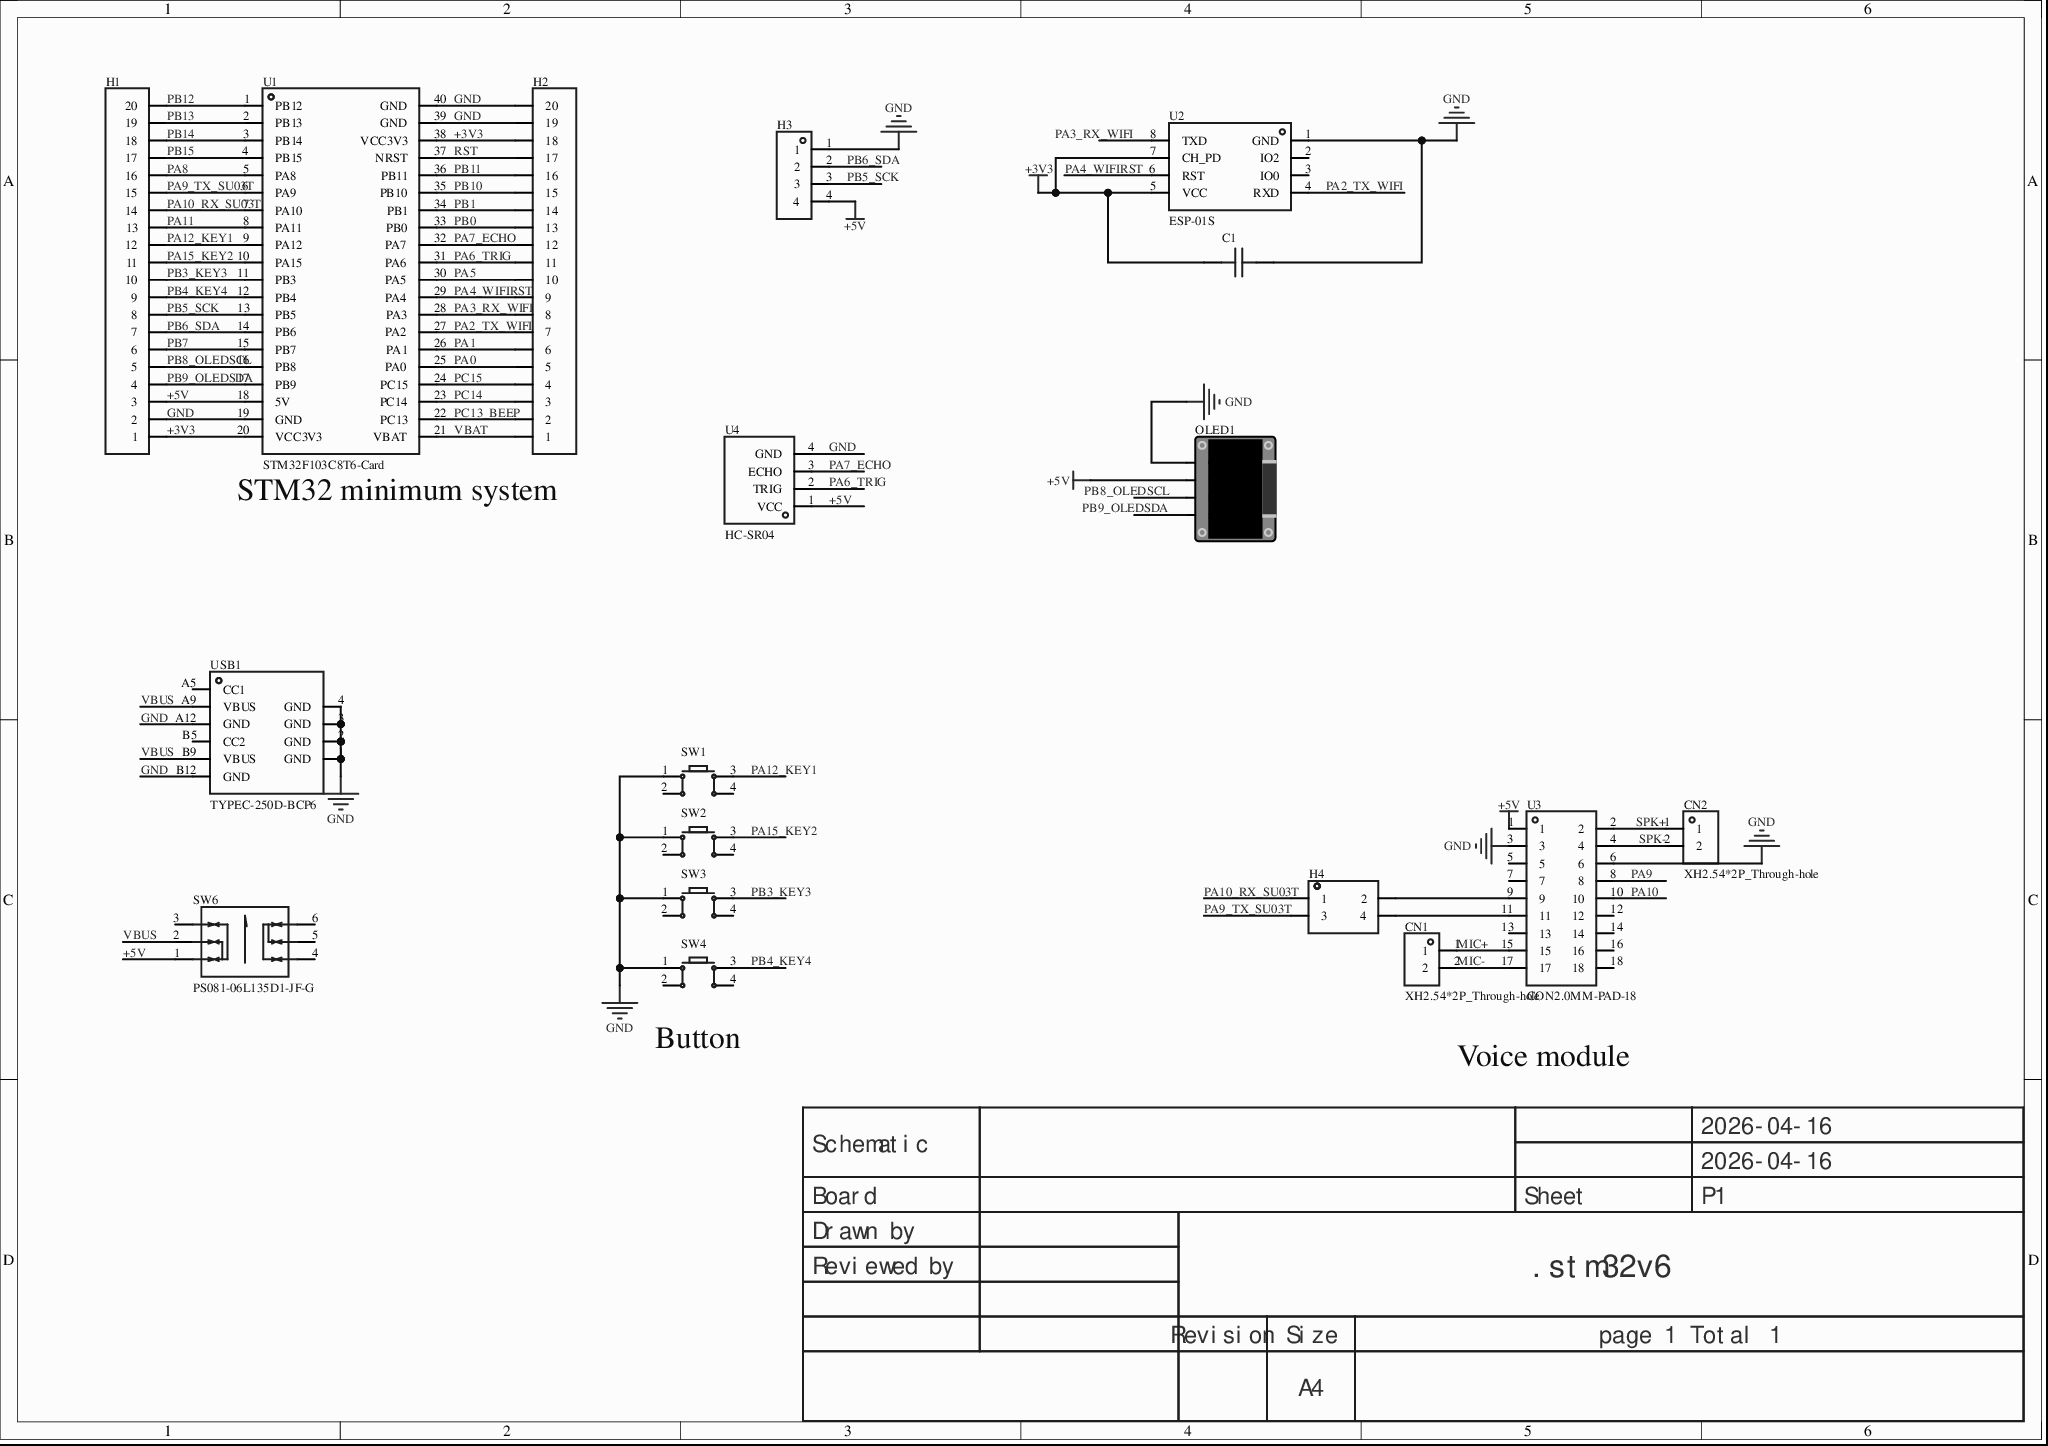
[diagram p0: MISC89113-3.schdoc]
# Altium project MISC89113-2.PrjPcb
1 sheet, 18 parts. Net scope: global (net labels, ports and power ports of the same name join across sheets).
Board file: MISC89113.pcbdoc

## Sheet MISC89113-3.schdoc
size 297 x 209 mm; Version: V1.0; @Project Name: MISC89113; @Page Count: 1; @Update Date: 2026-04-16; @Create Date: 2026-04-16; @Schematic Name: MISC89113; @Page No: 1; @Create Time: 23:22:16; @Update Time: 17:32:40; @Board Name: MISC89113

### Parts
C1  100nF  [C0603]  (value not drawn)
CN1  XH2.54*2P_Through-hole  [CONN-TH_2P-P2.50-XH2.54-2P]
CN2  XH2.54*2P_Through-hole  [CONN-TH_2P-P2.50-XH2.54-2P]
H1  (no value)  [HDR-TH_20P-P2.54-V-F]
H2  (no value)  [HDR-TH_20P-P2.54-V-F]
H3  (no value)  [HDR-TH_4P-P2.54-V-F]
H4  (no value)  [HDR-TH_4P-P2.54-V-F-R2-C2-S2.54]
OLED1  (no value)  [0.96OLED_4P]
SW1  (no value)  [SW-TH_4P-L6.0-W6.0-P4.50-LS6.5]
SW2  (no value)  [SW-TH_4P-L6.0-W6.0-P4.50-LS6.5]
SW3  (no value)  [SW-TH_4P-L6.0-W6.0-P4.50-LS6.5]
SW4  (no value)  [SW-TH_4P-L6.0-W6.0-P4.50-LS6.5]
SW6  PS081-06L135D1-JF-G  [SW-TH_6P-L8.0-W8.0-P2.50-TL]
U1  STM32F103C8T6-Card  [CONN-TH_L53.3-W22.9_STM32F103C8T6-CARD]
U2  ESP-01S  [WIFIM-TH_ESP-01S]
U3  CON2.0MM-PAD-18  [CONN-TH_18P-P2.00_C9900078766]
U4  HC-SR04  [TH_HC-SR04V]
USB1  TYPEC-250D-BCP6  [USB-C-SMD_TYPEC-250D-BCP6]

### Nets
+3V3: C1.1 H1.1 H2.18 U1.20(VCC3V3) U1.38(VCC3V3) U2.5(VCC) U2.7(CH_PD)
+5V: H1.3 H3.4 OLED1.2(VCC) SW6.1 U1.18(5V) U3.1 U4.1(VCC)
GND: C1.2 H1.2 H2.19 H2.20 H3.1 OLED1.1(GND) SW1.1 SW2.1 SW3.1 SW4.1 U1.19(GND) U1.39(GND) U1.40(GND) U2.1(GND) U3.3 U3.6 U4.4(GND) USB1.1(GND) USB1.2(GND) USB1.3(GND) USB1.4(GND) USB1.A12(GND) USB1.B12(GND)
MIC+: CN1.1 U3.15
MIC-: CN1.2 U3.17
PA0: H2.5 U1.25(PA0)
PA1: H2.6 U1.26(PA1)
PA2_TX_WIFI: H2.7 U1.27(PA2) U2.4(RXD)
PA3_RX_WIFI: H2.8 U1.28(PA3) U2.8(TXD)
PA4_WIFIRST: H2.9 U1.29(PA4) U2.6(RST)
PA5: H2.10 U1.30(PA5)
PA6_TRIG: H2.11 U1.31(PA6) U4.2(TRIG)
PA7_ECHO: H2.12 U1.32(PA7) U4.3(ECHO)
PA8: H1.16 U1.5(PA8)
PA9: U3.8
PA9_TX_SU03T: H1.15 H4.3 U1.6(PA9)
PA10: U3.10
PA10_RX_SU03T: H1.14 H4.1 U1.7(PA10)
PA11: H1.13 U1.8(PA11)
PA12_KEY1: H1.12 SW1.3 U1.9(PA12)
PA15_KEY2: H1.11 SW2.3 U1.10(PA15)
PB0: H2.13 U1.33(PB0)
PB1: H2.14 U1.34(PB1)
PB3_KEY3: H1.10 SW3.3 U1.11(PB3)
PB4_KEY4: H1.9 SW4.3 U1.12(PB4)
PB5_SCK: H1.8 H3.3 U1.13(PB5)
PB6_SDA: H1.7 H3.2 U1.14(PB6)
PB7: H1.6 U1.15(PB7)
PB8_OLEDSCL: H1.5 OLED1.3(SCL) U1.16(PB8)
PB9_OLEDSDA: H1.4 OLED1.4(SDA) U1.17(PB9)
PB10: H2.15 U1.35(PB10)
PB11: H2.16 U1.36(PB11)
PB12: H1.20 U1.1(PB12)
PB13: H1.19 U1.2(PB13)
PB14: H1.18 U1.3(PB14)
PB15: H1.17 U1.4(PB15)
PC13_BEEP: H2.2 U1.22(PC13)
PC14: H2.3 U1.23(PC14)
PC15: H2.4 U1.24(PC15)
RST: H2.17 U1.37(NRST)
SPK+: CN2.1 U3.2
SPK-: CN2.2 U3.4
VBAT: H2.1 U1.21(VBAT)
VBUS: SW6.2 USB1.A9(VBUS) USB1.B9(VBUS)
NetH4_2: H4.2 U3.9
NetH4_4: H4.4 U3.11

Not connected (* = marked no-connect by the designer): SW1 2 4; SW2 2 4; SW3 2 4; SW4 2 4; SW6 3 4 5 6; U2 2(IO2)* 3(IO0)*; U3 5 7 12 13 14 16 18; USB1 A5(CC1)* B5(CC2)*

### Notes on the sheet
- STM32 minimum system
- (near SW4) Button
- Voice module
- Labels drawn without touching a wire or pin: GND, VCC
- 2026-04-16
- Schematic
- Board
- Sheet
- P1
- Drawn by
- Reviewed by
- .stm32v6
- Revision
- Size
- A4
- page 1 Total 1

### Library data of the parts
C1 = CAP_0603: Symbol: Capacitance; ConvertToPcb: yes; ModelId: ac125912035d415993ca9572d50418b10819f05c4eef4c71ace90d822a990e87; ModelName: C0603_L1.6-W0.8-H0.8; ModelTransform: 62.992,31.496,0,0,0,0,0,0,0; Device: CAP_0603; AddInBom: yes; Supplier Footprint: 0603; FootprintName: C0603; Value: 100nF
CN1 CN2 = XH2.54*2P_直插: AddInBom: yes; ModelId: 325c595e30db4df8abe76612dd40b0fa0819f05c4eef4c71ace90d822a990e87; ModelTransform: 295.275,228.346,0,180,0,0,-0.002,-20.079,-137.795; Symbol: XH2.54*2P_Through-hole; Device: XH2.54*2P_Through-hole; LCSC Part Name: XH2.54*2P_直插; SupplierPart: C9900008615; ManufacturerPart: XH2.54*2P_直插; Supplier Footprint: XH2.54_2P; JLCPCB Part Class: Extended Part; Supplier: LCSC; ConvertToPcb: yes; FootprintName: CONN-TH_2P-P2.50-XH2.54-2P; ModelName: CONN-TH_2P-P2.50-XH2.54-2P
H1 H2 = HDR-F_2.54_1x20P: ConvertToPcb: yes; ModelId: db7015f7ad9d48b8a3b1188db02e3429; ModelName: HDR-F-2.54_1x20; ModelTransform: 1999.996,100,0,0,0,0,0,0,-118.11; Symbol: HDR-F_2.54_1x20P; Device: HDR-F_2.54_1x20P; AddInBom: yes; SupplierPart: C50984; Supplier Footprint: 插件; FootprintName: HDR-TH_20P-P2.54-V-F
H3 = HDR-F_2.54_1x4P: Symbol: 2.54-1*4P female; ConvertToPcb: yes; ModelId: d187812051054f85879fcaa51a310d8e0819f05c4eef4c71ace90d822a990e87; ModelTransform: 419.6842,98.464,0,0,0,0,0,0,-118.11; Device: HDR-F_2.54_1x4P; AddInBom: yes; SupplierPart: C2718488; Supplier Footprint: 插件; FootprintName: HDR-TH_4P-P2.54-V-F; ModelName: HDR-TH_4P-P2.54-V-F
H4 = HDR-F_2.54_2x2: Symbol: HDR-F-2.54_2x2; ConvertToPcb: yes; ModelId: 870c884146ee4765973edc845f10b7af0819f05c4eef4c71ace90d822a990e87; ModelName: HDR-TH_4P-P2.54-F-LI-2X2P; ModelTransform: 215.7476,196.85,0,0,0,0,0,0,-118.11; Device: HDR-F_2.54_2x2; AddInBom: yes; SupplierPart: C92273; Supplier Footprint: 插件; FootprintName: HDR-TH_4P-P2.54-V-F-R2-C2-S2.54
OLED1 = 0.96OLED模块_4P: Symbol: 0.96OLED module_4P; ConvertToPcb: yes; ModelId: 79c000fdb68d45a296c2e9bedf4f9055; ModelTransform: 1393.69792,1318.895,0,0,0,0,0,-560.079,-137.795; Device: 0.96OLED module_4P; AddInBom: yes; FootprintName: 0.96OLED_4P; Supplier Footprint: 插件; ModelName: 0.96OLED_4P
SW1-SW4 = Key_TH_6x6x6: Contact current: 50mA; rated voltage (DC): 12V; insulation resistance: 100MΩ; circuit structure: SPST; mounting: through-hole; button shape: round button; button/cap color: black; actuating force: 260gf@±30gf; operating temperature: -25℃~+70℃; pin style: PC pin; switch length: 6mm; switch width: 6mm; switch height: 6mm; with bracket: no;; Symbol: Tactile push button; AddInBom: yes; ModelId: 20eee248bc684ccd8cbdbb1d0d91ec6f0819f05c4eef4c71ace90d822a990e87; ModelName: SW-TH_4P-L6.0-W6.0-H5.0-LS6.5-P4.50; ModelTransform: 236.22,323.03,0,90,0,0,0,0,-137.795; Device: Key_TH_6x6x6; ConvertToPcb: yes; FootprintName: SW-TH_4P-L6.0-W6.0-P4.50-LS6.5; Supplier Footprint: 插件
SW6 = PS081-06L135D1-JF-G: Circuit structure: DPDT; self-lock/no-lock: self-lock; mounting: through-hole; contact current: 100mA; rated voltage: 30V;; Manufacturer: Khon(康宏电子); AddInBom: yes; ModelId: 81096a2982954f00b80aabbc3df69c720819f05c4eef4c71ace90d822a990e87; ModelTransform: 314.96394,314.96,0,90,0,0,0,0,-137.795; Actuator/Cap Color: Blue; Symbol: PS081-06L135D1-JF-G; Device: PS081-06L135D1-JF-G; LCSC Part Name: 8x8自锁开关; SupplierPart: C46533676; ManufacturerPart: PS081-06L135D1-JF-G; Supplier Footprint: DIP-6P,8x8mm; JLCPCB Part Class: Extended Part; Datasheet: https://item.szlcsc.com/datasheet/PS081-06L135D1-JF-G/48661190.html; Supplier: LCSC; ConvertToPcb: yes; FootprintName: SW-TH_6P-L8.0-W8.0-P2.50-TL; ModelName: SW-TH_6P-L8.0-W8.0-P2.50-TL; Circuit: DPDT; Self Lock / No Lock: Self-lock; Mounting Type: Through-hole; Contact Current: 100mA; Voltage Rating: 30V; Termination Style: PC pin; Operating Temperature: -25℃~+70℃
U1 = STM32F103C8T6-Card: AddInBom: yes; Symbol: STM32F103C8T6-CARD; Device: STM32F103C8T6-Card; LCSC Part Name: STM32F103C8T6-Card; SupplierPart: C9900077949; ManufacturerPart: STM32F103C8T6-Card; Supplier Footprint: 插件; Supplier: LCSC; ConvertToPcb: yes; FootprintName: CONN-TH_L53.3-W22.9_STM32F103C8T6-CARD
U2 = ESP-01S_C111009: AddInBom: yes; ModelId: eb7175da78ae48b3b1568cfe3027405f0819f05c4eef4c71ace90d822a990e87; ModelTransform: 582.676,976.37608,0,0,0,0,0,388.346,-118.11; Symbol: ESP-01S; Device: ESP-01S_C111009; LCSC Part Name: ESP-01S; SupplierPart: C111009; ManufacturerPart: ESP-01S; Supplier Footprint: -; JLCPCB Part Class: Extended Part; Supplier: LCSC; ConvertToPcb: yes; FootprintName: WIFIM-TH_ESP-01S; ModelName: WIFIM-TH_ESP-01S
U3 = CON2.0MM-PAD-18: AddInBom: yes; ModelId: 07100c6dd3a4442ea12d6f5a4e41c4c80819f05c4eef4c71ace90d822a990e87; ModelTransform: 787.7937,374.015,0,0,0,0,0,-14.961,-118.11; Symbol: CON2.0MM-PAD-18; Device: CON2.0MM-PAD-18; LCSC Part Name: CON2.0MM-PAD-18; SupplierPart: C9900078766; ManufacturerPart: CON2.0MM-PAD-18; Supplier Footprint: TH-2*9P-2.0; JLCPCB Part Class: Extended Part; Supplier: LCSC; ConvertToPcb: yes; FootprintName: CONN-TH_18P-P2.00_C9900078766; ModelName: CONN-TH_18P-P2.00_C9900078766
U4 = HC-SR04: Manufacturer: Universal Microelectronics; AddInBom: yes; Symbol: HC-SR04; Device: HC-SR04; LCSC Part Name: HC-SR04; SupplierPart: C19857336; ManufacturerPart: HC-SR04; Supplier Footprint: -; JLCPCB Part Class: Extended part; Datasheet: https://atta.szlcsc.com/upload/public/pdf/source/20240122/47B8E374E428935B7962A2189EF91AAC.pdf; Supplier: LCSC; ConvertToPcb: yes; FootprintName: TH_HC-SR04V
USB1 = TYPEC-250D-BCP6: Connector type: Type-C; standard: USB 3.1; gender: female; number of ports: 1; number of contacts: 6P; mounting: SMD flat; rated current - power: 3A; operating temperature range: -25℃~+85℃; soldering temperature (max): 260℃;; Manufacturer: XUNPU(讯普); AddInBom: yes; ModelId: 3327e6c5ea684c7f81f0821c55fd3a350819f05c4eef4c71ace90d822a990e87; ModelTransform: 351.9678,275.59,0,0,0,0,-0.005,-47.555,-39.37; Number of Ports: 1; Symbol: TYPEC-250D-BCP6; Device: TYPEC-250D-BCP6; LCSC Part Name: Type-C 母 卧贴; SupplierPart: C720626; ManufacturerPart: TYPEC-250D-BCP6; Supplier Footprint: SMD; JLCPCB Part Class: Extended Part; Datasheet: https://atta.szlcsc.com/upload/public/pdf/source/20200812/C720626_0B3D9525FB9C6D818696E28704B18234.pdf; Supplier: LCSC; ConvertToPcb: yes; FootprintName: USB-C-SMD_TYPEC-250D-BCP6; ModelName: USB-C-SMD_TYPEC-250D-BCP6; Connector Type: Type-C; Standard: USB 3.1; Gender: Female; Number of Contacts: 6P; Mounting Style: SMD flat; Current Rating - Power (Max): 3A; Operating Temperature Range: -25℃~+85℃; Welding Temperature (Max): 260℃